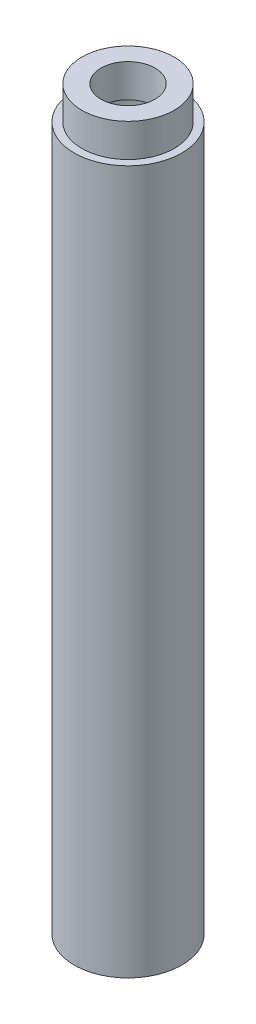
from build123d import *


with BuildPart() as part:
    # Sketch1 → Revolve1 (revolve)
    with BuildSketch(Plane.XY, mode=Mode.PRIVATE) as revolve1_sk:
        Polygon((-2.45, 29.940117832), (-2.45, -2.059882168), (-2.35, -2.059882168), (-2.35, 29.740117832), (-1.883917375, 29.740117832), (-1.883917375, 29.940117832), (-1.23, 29.940117832), (-1.23, 31.44696074), (-2.1, 31.44696074), (-2.1, 29.940117832), align=None)
    revolve(revolve1_sk.sketch.rotate(Axis((0, -5.459851486, 0), (0, 1, 0)), 270), axis=Axis((0, -5.459851486, 0), (0, 1, 0)))


solid = part.part
